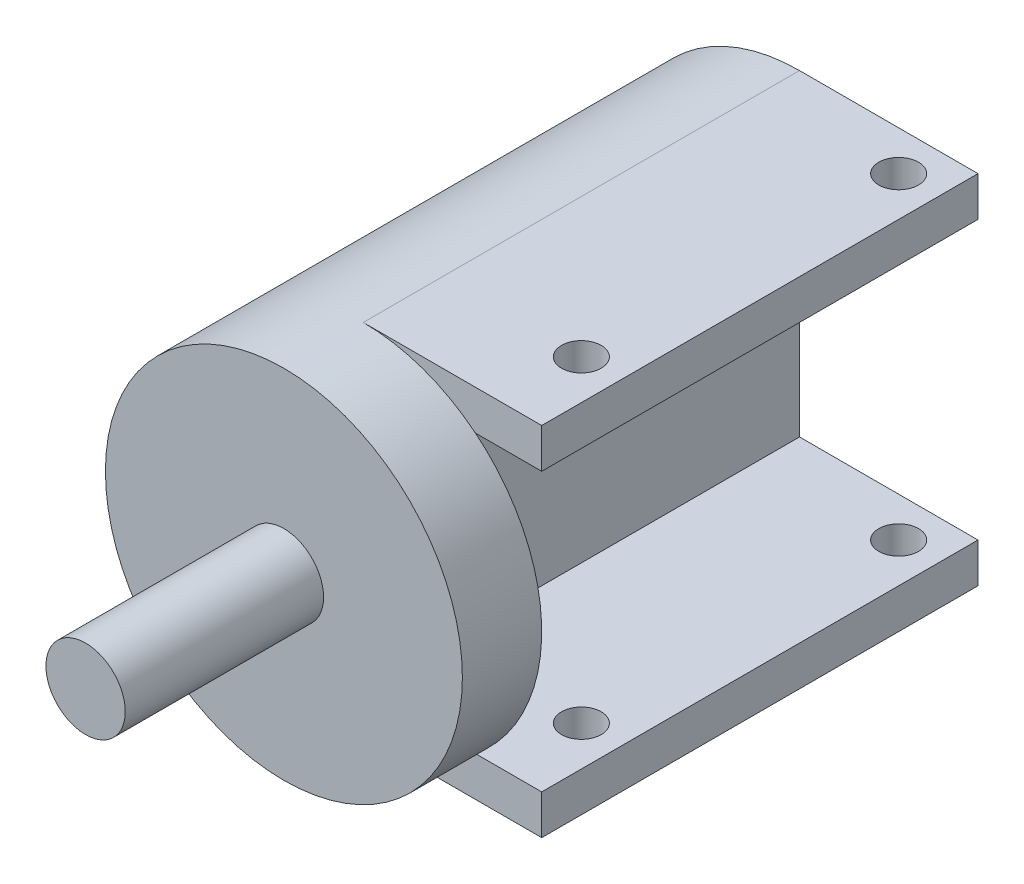
SolidWorks part; units mm, degrees
ref_plane "前视" through (0, 0, 0) normal (0, 0, 1) x (1, 0, 0)
ref_plane "上视" through (0, 0, 0) normal (0, 1, 0) x (1, 0, 0)
ref_plane "右视" through (0, 0, 0) normal (1, 0, 0) x (0, 0, -1)
sketch "草图1" plane through (0, 0, 0) normal (0, 0, 1) x (1, 0, 0)
  circle A0 centre (0, 0) radius 22.5
extrude "凸台-拉伸1" add sketch "草图1" along normal blind 65
sketch "草图2" plane through (0, 0, 65) normal (0, 0, 1) x (1, 0, 0)
  circle A0 centre (0, 0) radius 5
extrude "凸台-拉伸2" add sketch "草图2" along normal blind 25
ref_plane "基准面1" through (0, 22.5, 0) normal (0, 1, 0) x (-1, 0, 0)
sketch "草图3" plane through (0, 22.5, 0) normal (0, 1, 0) x (-1, 0, 0)
  line L0 (0, 0) -> (0, 55)
  line L1 (0, 0) -> (-22.5, 0)
  line L3 (0, 55) -> (-22.5, 55)
  line L4 (-22.5, 0) -> (-22.5, 55)
  dimension "D1" = 55
extrude "凸台-拉伸3" add sketch "草图3" against normal blind 5
ref_plane "基准面2" through (0, -22.5, 0) normal (0, 1, 0) x (-1, 0, 0)
sketch "草图4" plane through (0, -22.5, 0) normal (0, 1, 0) x (-1, 0, 0)
  line L0 (-22.5, 65) -> (-22.5, 0) construction
  line L1 (0, 0) -> (-22.5, 0)
  line L2 (0, 0) -> (0, 55)
  line L3 (0, 55) -> (-22.5, 55)
  line L4 (-22.5, 0) -> (-22.5, 55)
  dimension "D1" = 55
extrude "凸台-拉伸4" add sketch "草图4" along normal blind 5
sketch "草图5" plane through (0, 0, 0) normal (0, 0, -1) x (-1, 0, 0)
  line L0 (-14.1421, -17.5) -> (0, -17.5)
  line L1 (0, -17.5) -> (0, 17.5)
  line L2 (0, 17.5) -> (-14.1421, 17.5)
  line L6 (-14.1421, -17.5) -> (-22.5, -17.5)
  line L7 (-22.5, -17.5) -> (-22.5, -22.5)
  line L8 (-22.5, -22.5) -> (0, -22.5)
  line L9 (0, 22.5) -> (-22.5, 22.5)
  line L10 (-22.5, 22.5) -> (-22.5, 17.5)
  line L11 (-22.5, 17.5) -> (-14.1421, 17.5)
  arc A2 (-14.1421, 17.5) -> (-14.1421, -17.5) centre (0, 0) ccw
  arc A3 (0, -22.5) -> (0, 22.5) centre (0, 0) ccw
  arc A4 (-14.1421, 17.5) -> (-14.1421, -17.5) centre (0, 0) ccw
  dimension "D1" = 0
extrude "切除-拉伸1" cut sketch "草图5" against normal blind 55
sketch "草图6" plane through (0, -22.5, 0) normal (0, -1, 0) x (1, 0, 0)
  line L0 (22.5, 55) -> (22.5, 0) construction
  line L1 (22.5, 0) -> (0, 0) construction
  line L2 (0, 55) -> (22.5, 55) construction
  circle A0 centre (17.5, 5) radius 2.5
  circle A1 centre (17.5, 45) radius 2.5
  dimension "D1" = 5
  dimension "D2" = 5
  dimension "D3" = 5
  dimension "D4" = 5
  dimension "D5" = 5
  dimension "D6" = 10
extrude "切除-拉伸2" cut sketch "草图6" against normal blind 60
